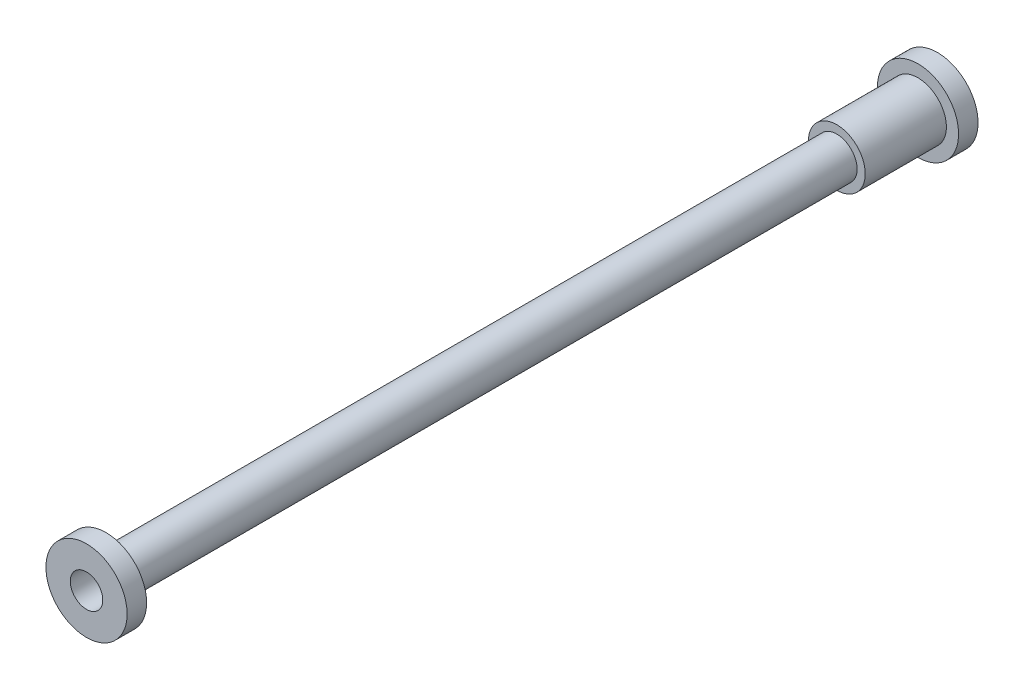
from build123d import *

# Parameters (mm, degrees)
SKETCH1_R           = 12.5
BOSS_EXTRUDE1_DEPTH = 450
SKETCH2_R           = 17.5
BOSS_EXTRUDE2_DEPTH = 50
SKETCH3_R           = 25
BOSS_EXTRUDE3_DEPTH = 12
BOSS_EXTRUDE4_START = 12
SKETCH4_R           = 25
BOSS_EXTRUDE4_DEPTH = 12
SKETCH5_R           = 10
CUT_EXTRUDE1_DEPTH  = 526.191393684


with BuildPart() as part:
    # Sketch1 → Boss-Extrude1 (new body)
    with BuildSketch(Plane.XY):
        Circle(SKETCH1_R)
    extrude(amount=BOSS_EXTRUDE1_DEPTH)

    # Sketch2 → Boss-Extrude2 (add)
    with BuildSketch(Plane(origin=(0, 0, 0), x_dir=(-1, 0, 0), z_dir=(0, 0, -1))):
        Circle(SKETCH2_R)
    extrude(amount=BOSS_EXTRUDE2_DEPTH)

    # Sketch3 → Boss-Extrude3 (add)
    with BuildSketch(Plane(origin=(0, 0, -50), x_dir=(-1, 0, 0), z_dir=(0, 0, -1))):
        Circle(SKETCH3_R)
    extrude(amount=BOSS_EXTRUDE3_DEPTH)

    # Sketch4 → Boss-Extrude4 (add)
    with BuildSketch(Plane.XY.offset(450).offset(BOSS_EXTRUDE4_START)):
        with Locations(Location((0, 0, 0), (0, 0, 180))):
            Circle(SKETCH4_R)
    extrude(amount=-BOSS_EXTRUDE4_DEPTH)

    # Sketch5 → Cut-Extrude1 (cut, through all)
    with BuildSketch(Plane.XY.offset(462)):
        Circle(SKETCH5_R)
    extrude(amount=-CUT_EXTRUDE1_DEPTH, mode=Mode.SUBTRACT)


solid = part.part
